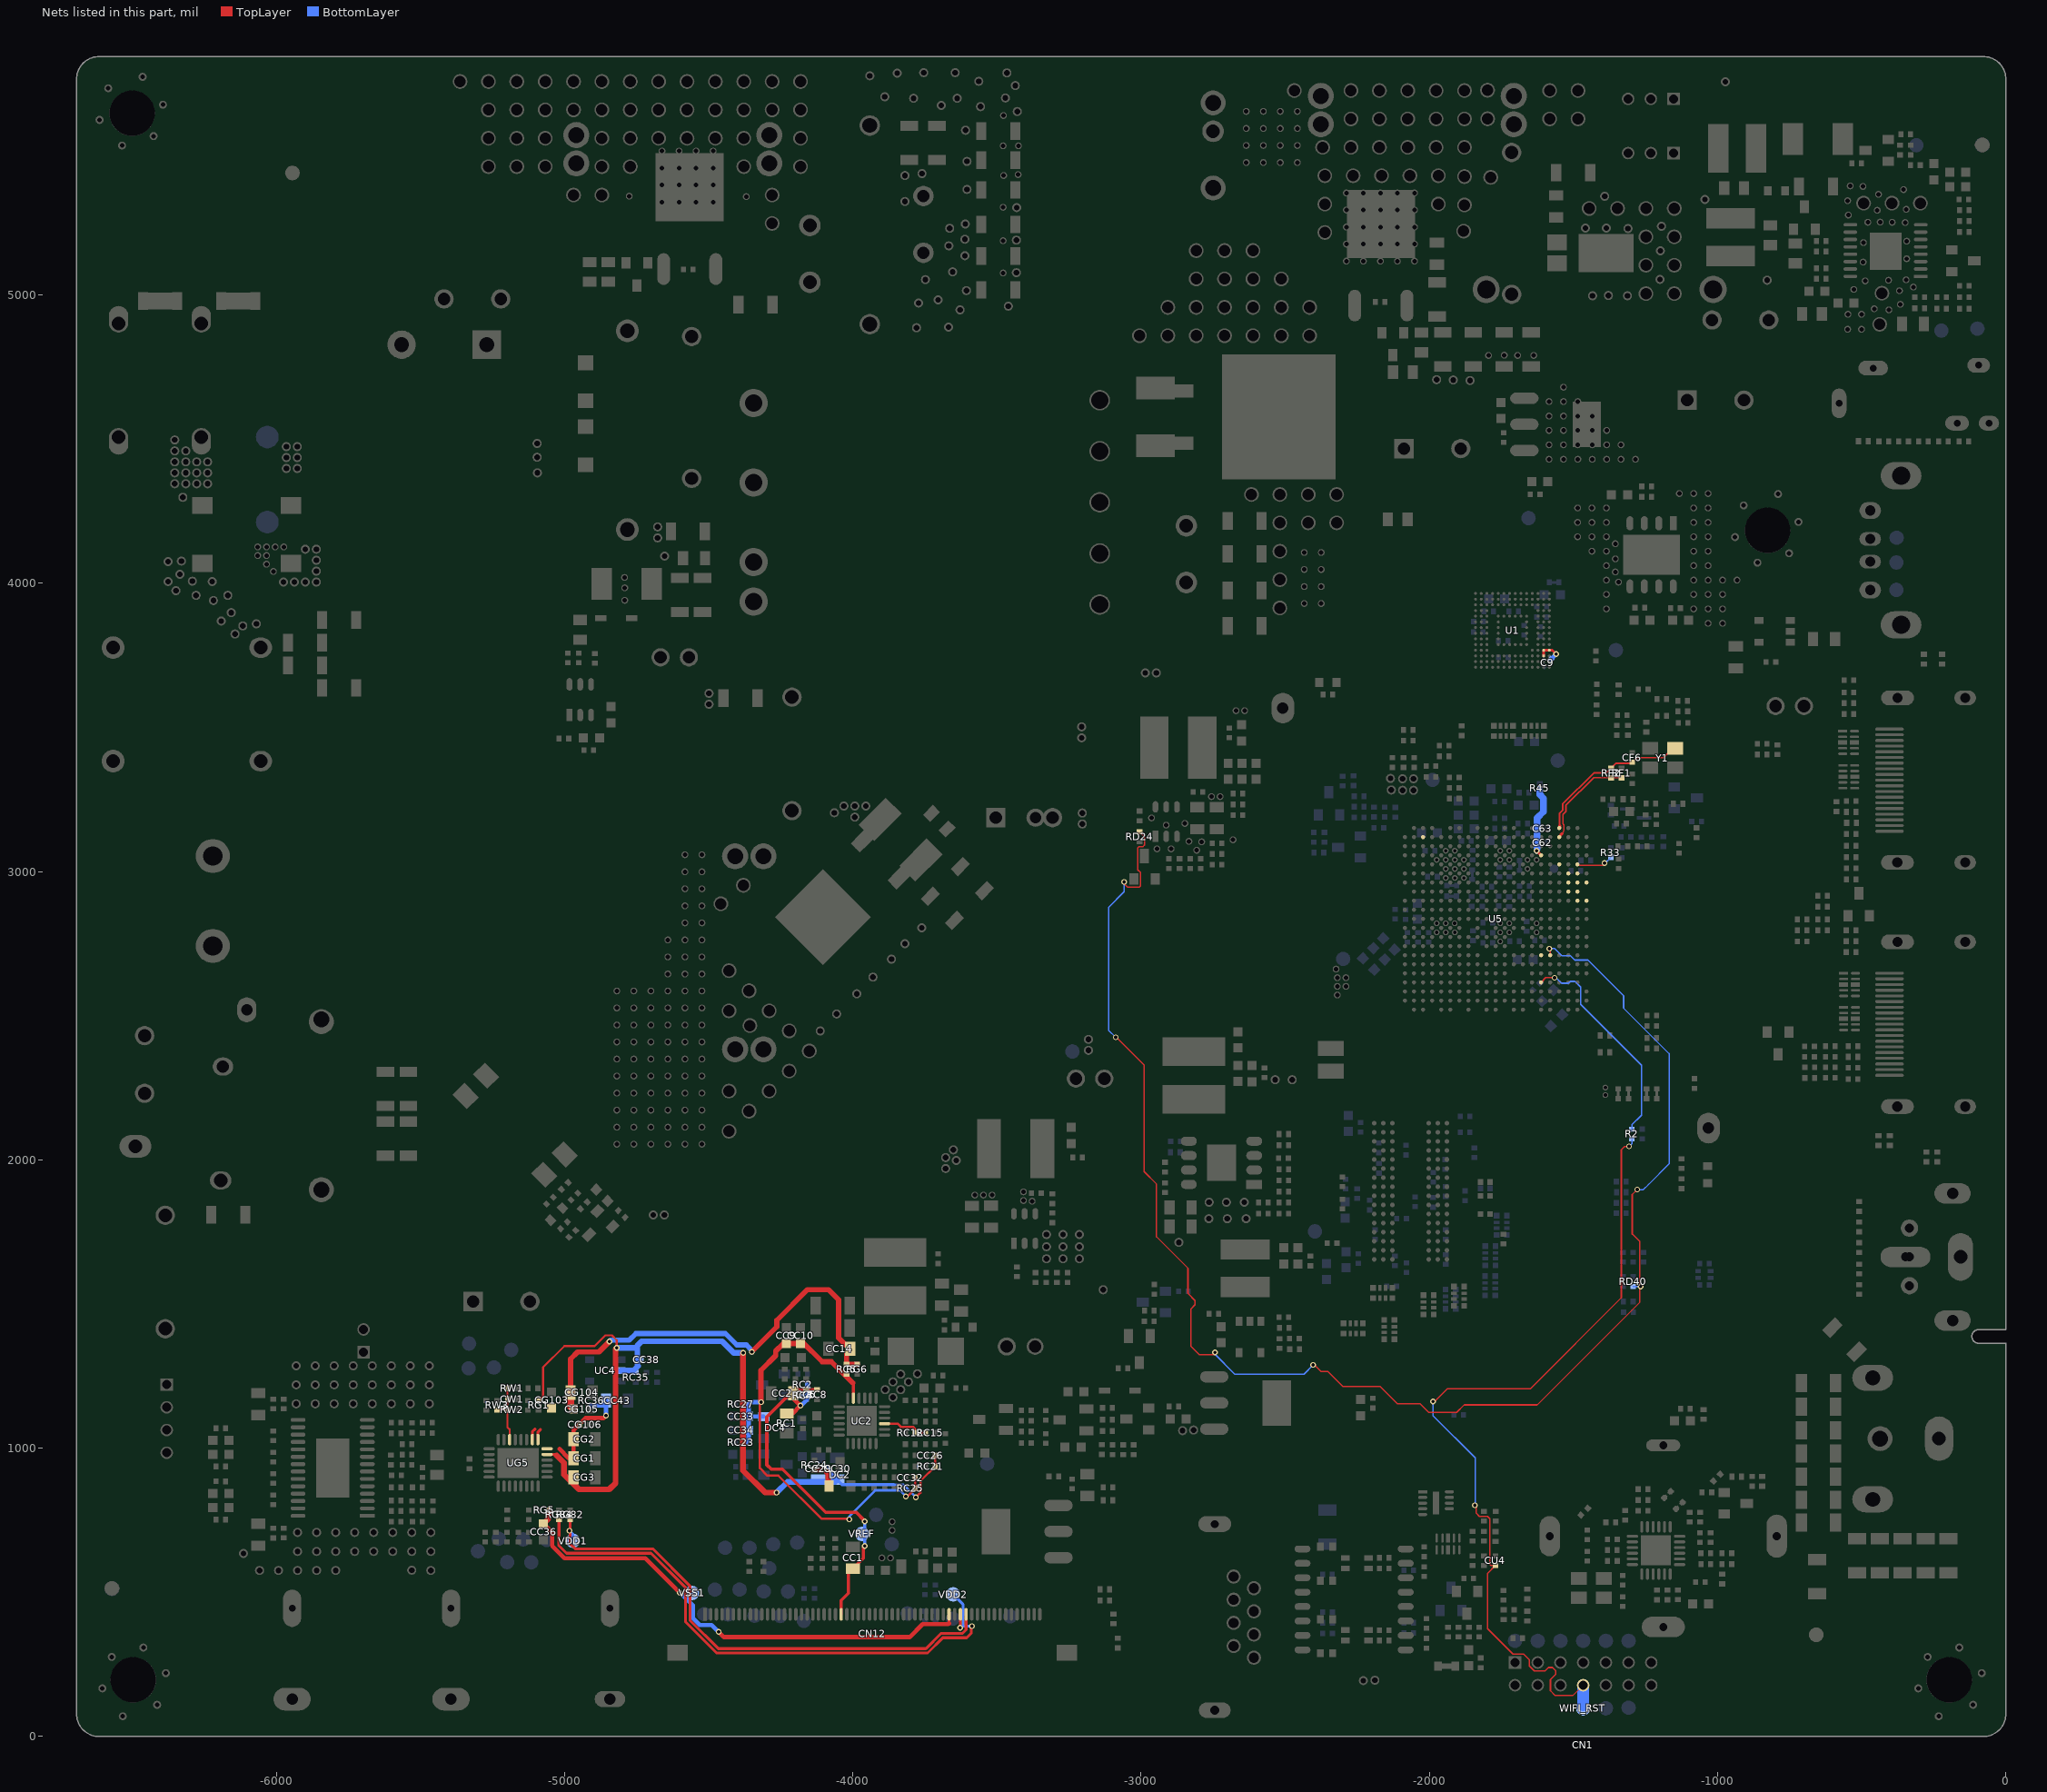
[diagram p0: the nets of this part, all layers, seen from the top]
# Altium PCB MISC84395.PcbDoc (part 24 of 26)
Units mil, origin at the board's own origin, x right, y up, seen from the top; angles counter-clockwise.
Board outline 6692.91 x 5826.77 mil, 2 copper layers (TopLayer, BottomLayer), stack 61.855 mil thick; 951 components, 565 nets, 4374 pads, 1804 vias.
Unrouted connection lines stored in the file: 1.

## Via types
v1: diameter 19.68, hole 11.81, TopLayer to BottomLayer, tented both sides, 1262 vias
v2: diameter 23.62, hole 15.75, TopLayer to BottomLayer, tented both sides, 524 vias
v3: diameter 31.5, hole 19.68, TopLayer to BottomLayer, tented both sides, 11 vias
v4: diameter 24, hole 16, TopLayer to BottomLayer, tented both sides, 6 vias
v5: diameter 19, hole 11.81, TopLayer to BottomLayer, tented both sides, 1 vias

## Nets (pads, with @x,y where several pads share a name; then routed paths per layer and width w, separated by ;. In a path a pad name is that pad's centre, name@x,y a point inside that pad or via, vN(x,y) a via of type N, cw(c..) or ccw(c..) an arc to the next point about the centre after c; other vN are vias at no path point) (continued)
VDD1: CN12.47 RG82.1 VDD1.1 | length 1792.2
  TopLayer w10: RG82.1@-4981,752.27 -4981,669 -4963,651 -4693.79,651 -4564.84,522.06 -4564.84,403.3 -4466.55,305 -3746.5,305 -3693.76,357.74 -3619.78,357.74 -3607.2,370.32 CN12.47@-3607.2,418.08
  BottomLayer w10: v1(-4983,714) -4971,702 VDD1.1@-4971,679
VDD2: CN12.46 RG84.1 VDD2.1 | length 2001
  TopLayer w10: RG84.1@-5019,752.27 -5019,661.75 -4993.25,636 -4700,636 -4579.84,515.84 -4579.84,397.08 -4472.76,290 -3740.29,290 -3687.54,342.74 -3604.76,342.74 -3589,358.5 -3589,381 v1(-3587,383) ; v1@-3626.89,377.59 CN12.46@-3626.89,418.08
  BottomLayer w10: VDD2.1@-3652,493 -3618,459 -3618,386.47 ; v1@-3626.89,377.59 -3621.47,383 v1(-3587,383)
  other v1: -3628,377.59
VDDI: C9.1 U1.C2 U1.D1 U1.D2 | length 98.1
  TopLayer w9.8: U1.C2@-1603.6,3747.97 U1.D2@-1603.6,3767.66 U1.D1@-1583.91,3767.66 -1573.52,3767.66 v1(-1560.21,3754.34)
  BottomLayer w9.8: v1@-1563.71,3750.84 v1(-1560.21,3754.34)
  BottomLayer w15: C9.1@-1577.17,3736.83 -1560.21,3753.8 v1(-1560.21,3754.34)
VDDP_EMMC: C62.2 C63.2 R45.2 R45.3 U5.V6 | length 245.6
  TopLayer w10: v1(-1628.24,3072.3) U5.V6@-1612.49,3056.56
  BottomLayer w19.68: v1(-1628.24,3072.3) -1626.27,3074.27 v1@-1626.27,3078.21
  BottomLayer w23.62: v1@-1626.27,3078.21 -1626.27,3185.65 -1603.63,3208.29 -1603.63,3253.71 -1617.27,3267.35 R45.2@-1617.27,3272.01 R45.2@-1617.27,3279.8
VDET1: CW1.2 RW1.2 RW2.2 RW3.2 UG5.6 | length 217.3
  TopLayer w7: RW3.2@-5236,1135.27 RW2.2@-5200,1135.27 ; RW1.2@-5197.73,1208 CW1.2@-5197.73,1170 RW2.2@-5197.73,1133 -5197.73,1072.11 -5190.53,1064.91 UG5.6@-5190.53,1029.71
VDIV: RC12.2 RC15.1 UC2.15 | length 162.9
  TopLayer w8: UC2.15@-3890,1085.08 -3845.08,1085.08 -3834,1074 -3791,1074 -3784.27,1067.27 RC12.2@-3784.27,1054 RC15.1@-3747.73,1054
VGA_B_IN_IC: U5.P3
VGA_COM_IN_IC: U5.R3
VGA_G_IN_IC: U5.P2
VGA_HS_IN_IC: U5.N1
VGA_R_IN_IC: U5.R2
VGA_VS_IN_IC: U5.N2
VGH: CC9.1 CC10.1 CC32.2 CC33.2 CC34.2 DC4.3 RC5.2 RC23.2 RC25.2 RC27.2 UC2.23 | length 1841.2
  TopLayer w8: v1@-4317.66,1164 -4318.5,1163.16 -4322,1159.66 -4322,931 -4296,905 -4258,905 -4108,755 -4014,755 v1(-4012,753) ; v1(-3816,833) -3810.06,833 -3784.26,858.8 CC32.2@-3784.26,898
  TopLayer w10: -4000.58,1226.57 -3998.27,1224.26 UC2.23@-3998.27,1173.66
  TopLayer w18: v1@-4318.5,1159.66 v1@-4318.5,1160.5 ; v1(-4317.66,1159.66) v1@-4318.5,1160.5 ; CC10.1@-4181,1363.19 CC9.1@-4231,1363.19 -4240.97,1363.19 -4267.37,1336.79 -4267.37,1321.51 -4318.5,1270.38 -4318.5,1163.16 v1@-4318.5,1160.5 ; CC10.1@-4181,1367.25 -4174.44,1367.25 CC10.1@-4175.37,1368.19 ; CC10.1@-4181,1368.19 CC10.1@-4175.37,1368.19 ; CC10.1@-4173.65,1368.19 CC10.1@-4174.65,1368.19 ; -4000.58,1226.57 -4074.01,1300 -4106.46,1300 CC10.1@-4174.65,1368.19 ; CC10.1@-4175.37,1368.19 CC10.1@-4174.65,1368.19
  BottomLayer w8: v1(-4012,753) -4012,764 -3922,854 -3836,854 -3816,834 v1(-3816,833)
  BottomLayer w15: RC23.2@-4372.27,1020.19 -4361.19,1031.27 ; CC34.2@-4361.19,1062.19 -4361.19,1031.27 ; v1@-4319.66,1160 -4352,1160 -4361.19,1150.81 -4361.19,1126 ; DC4.3@-4316.16,1110 DC4.3@-4318.77,1110 ; DC4.3@-4309.5,1110.19 CC33.2@-4361.19,1110.19 -4361.19,1126 ; -4361.19,1031.27 -4361.19,1126 ; DC4.3@-4318.77,1110 -4321.77,1110 -4320.27,1108.5 DC4.3@-4318.77,1110
VGHM: CC14.2 CG103.2 CG104.1 CG105.2 RC5.1 RG6.2 UG5.1 UG5.2@-5111.79,1029.71 | length 1665.2
  TopLayer w10: UG5.2@-5111.79,1029.71 -5111.79,1057.21 -5103,1066 ; UG5.1@-5092.1,1029.71 -5092.1,1056.9 -5084,1065
  TopLayer w18: -4979,1164 CG104.1@-4979,1193 -4979,1221 ; -4979,1245.18 -4979,1221 ; v1(-4844.5,1370) -4880.5,1334 -4954.5,1334 -4979,1309.5 -4979,1221 ; v1@-4350.54,1334.54 -4263.75,1421.33 -4263.75,1443.75 -4157.87,1549.63 -4083.63,1549.63 -4049,1515 -4049,1382.49 -4011.51,1345 CC14.2@-4009,1345 ; CC14.2@-4012.75,1341.25 -4011.51,1340 -4009,1340 -4022,1327 RC5.1@-4022,1290.73 RG6.2@-3985,1290.73
  TopLayer w25: CG105.2@-4979,1144 -4979,1164
  BottomLayer w18: v1(-4844.5,1370) -4839.5,1375 -4775.5,1375 -4752.5,1398 -4442,1398 -4402,1358 -4369.32,1358 -4350,1338.68 v1(-4350,1334)
VGL: CC26.2 CC29.1 CC30.1 CC38.1 CG3.1 DC2.1 RC21.2 RC24.2 RC35.2 RG1.1 UC4.2 UG5.27 | length 3244.4
  TopLayer w7: RG1.1@-5090,1165.73 -5074.08,1181.65 -5074.08,1280.91 -5000.49,1354.5 -4895.37,1354.5 -4859.18,1390.68 -4858.52,1391.34 -4835.66,1391.34 -4819,1374.68 v1(-4819,1348)
  TopLayer w8: v1(-3781,830) -3765,846 -3765,886.27 RC21.2@-3714.27,937 CC26.2@-3714.26,975
  TopLayer w10: UG5.27@-5060.61,978.53 -5023.67,978.53
  TopLayer w20: -5027.21,974.99 -5001.75,949.53 -5001.75,908.75 -4950,857 -4845,857 -4823,879 -4823,1344 v1(-4819,1348) ; v1(-4380.5,1331) -4380.5,922.78 -4303.85,846.13 v1(-4264.65,846.13) ; RC24.2@-4133,925 v1@-4101,925 ; v1(-4099,927) -4085.5,913.5 DC2.1@-4085.5,869
  BottomLayer w8: -3858,874 -3825,874 v1(-3781,830)
  BottomLayer w10: CC30.1@-4055,891 -4038,874 -3858,874
  BottomLayer w20: v1(-4819,1348) -4755.5,1348 ; UC4.2@-4804.87,1269.73 -4760.27,1269.73 -4744.81,1285.19 ; -4747.5,1287.88 -4747.5,1356 -4732.5,1371 -4453.18,1371 -4413.18,1331 v1(-4380.5,1331) ; v1@-4263.87,846.13 -4226.37,883.63 CC30.1@-4061.37,883.63 ; v1(-4099,927) -4091,927 -4055,891 CC30.1@-4061.37,891
VGPIN1: U5.Y19
VID0_OUT_IC: RD24.2 RD40.1 U5.G5 | length 5527.1
  TopLayer w5: v1@-3084.53,2424 -2989.5,2328.97 -2989.5,1959.16 -2946.5,1916.16 -2946.5,1733.36 -2837.5,1624.36 -2837.5,1537.03 -2812.66,1512.18 -2812.66,1497.82 -2827.5,1482.97 -2827.5,1353.73 -2798.27,1324.5 v1@-2744,1324.5 ; v1@-3059,2958 -3047,2946 -3005.9,2946 -3002.25,2949.65 -3002.25,2996.98 -3011.25,3005.98 -3011.25,3082.3 -3006.85,3086.69 -2993.27,3086.69 -2987.66,3092.3 -2987.66,3120.39 RD24.2@-3005,3137.73 ; v1(-2403,1289.16) -2398.68,1289.16 -2375.18,1265.66 -2351.59,1265.66 -2299.54,1213.61 -2169.89,1213.61 -2109.89,1153.61 -2031.42,1153.61 ; -2098.2,1153.61 -2031.42,1153.61 ; U5.G5@-1580.99,2710.1 v1@-1580.99,2732.09 ; -1296.17,1742.86 -1296.17,1879.83 v1@-1280,1896 ; -1295.67,1742.86 -1269.65,1716.84 -1269.65,1510.04 -1269.65,1506.62 -1625.92,1150.34 -1879.01,1150.34 -1905.01,1124.34 -2002.15,1124.34 -2031.42,1153.61
  BottomLayer w5: v1(-3088,2425) -3113,2450 -3113,2875.47 -3058.66,2929.82 v1@-3058.66,2963.66 ; v1(-2744,1332) -2744,1326.13 -2674.87,1257 -2435.16,1257 v1(-2403,1289.16) ; v1@-1581.65,2732.74 -1565.17,2732.74 -1540.94,2708.51 ; -1541.26,2708.51 -1540.94,2708.51 ; -1540.83,2708.4 -1540.94,2708.51 ; RD40.1@-1293.22,1561.31 v1@-1267.31,1561.31 ; v1@-1280,1896 v1@-1279,1896 ; v1(-1279,1897) -1257.8,1897 -1239.9,1914.9 -1168.3,1986.5 -1168.3,2368.3 -1326.3,2526.3 -1326.3,2569.45 -1449.86,2693.01 -1495.91,2693.01 -1511.41,2708.51 -1540.94,2708.51
  other v1: -1267,1561 -1583.65,2732.74 -3059,2964
VID1_OUT_IC: U5.G6
VREF: CC1.2 CC2.2 CC5.1 CN12.25 RC1.2 RC2.2 RC4.2 RC4.3 RC8.1 VREF.1 | length 1324.8
  TopLayer w11: CN12.25@-4040.27,423.98 -4040.27,471.73 -4015,497 -4015,579 -4008,586 CC1.2@-4002,586 ; CC1.2@-4000,571 CC1.2@-3996,571 ; CC1.2@-4000,581.97 -3963,618.97 v1@-3963,657 ; v1(-3959,746) v1@-3959,748.01
  TopLayer w12: CC2.2@-4221,1186 -4298.5,1108.5 -4298.5,942.6 -4283.03,927.13 -4243.83,927.13 -4094.29,777.59 -3987.87,777.59 -3959,748.72 v1@-3959,748.01
  TopLayer w15: RC1.2@-4229,1120.09 -4209.91,1120.09 v1(-4182,1148) -4207,1173 CC2.2@-4207,1191 ; CC2.2@-4196.27,1201.73 -4162,1201.73 RC8.1@-4124,1201.73
  BottomLayer w11: v1(-3959,661) v1(-3959,746)
  BottomLayer w15: v1@-4178.6,1148 -4157.24,1169.36 RC2.2@-4157.24,1221
VSS: CC43.2 CG1.1 CG2.1 CG106.2 RC36.2 UG5.28 | length 385
  TopLayer w15: -5017.89,997.49 -4985.39,965 CG1.1@-4969.03,965 CG2.1@-4969.03,1031 -4969.03,1062.62 -4927.31,1104.34 -4864.66,1104.34 v1(-4856.03,1112.97)
  BottomLayer w15: RC36.2@-4906.73,1147.99 -4902,1147.99 CC43.2@-4867.25,1147.99 ; v1(-4856.03,1112.97) CC43.2@-4856.03,1164.73
VSS1: CC36.1 CN12.44 RG5.1 VSS1.1 | length 1722.9
  TopLayer w10: -3666.26,392 CN12.44@-3666.26,418.08
  TopLayer w15: CC36.1@-5073,737.81 -5043,707.81 -5043,661 -5000.5,618.5 -4719.5,618.5 v1(-4600,499) ; v1(-4465.59,363.22) -4447.37,345 -3802.6,345 -3757.77,389.83 -3668.43,389.83 -3666.26,392
  TopLayer w18: CC36.1@-5073,737.81 -5055.27,755.54 RG5.1@-5055.27,785
  BottomLayer w15: v1(-4600,499) -4599,499 -4555,455 -4555,410.74 -4531.25,386.99 -4489.36,386.99 v1(-4465.59,363.22)
WIFI_HOST_WAKE_IC: U5.U4
WIFI_PWR_EN_IC: R33.2 U5.U2 | length 123.6
  TopLayer w5: U5.U2@-1486.5,3025.06 -1483.41,3021.97 v1@-1392.04,3021.97
  BottomLayer w5: v1@-1390.36,3029.3 R33.2@-1370.65,3049.01
  other v1: -1392.04,3029.3
WIFI_RESET: CN1.8 CU4.2 R2.1 WIFI_RST.1 | length 2891.7
  TopLayer w5: v1(-1987,1162) -1982,1162 -1937.36,1206.64 -1649.41,1206.64 -1334.17,1521.88 -1334.17,2035.14 -1322.64,2046.67 v1(-1306.95,2046.67) ; v1(-1842,802) -1838,798 -1838,775 -1826.63,763.63 -1798.05,763.63 -1790.34,755.92 -1790.34,597 -1786.61,593.26 CU4.2@-1771,593.26 -1798.25,566.01 -1798.25,374.11 -1710.03,285.89 -1672.89,285.89 -1653.17,266.17 -1653.17,244.66 -1636.09,227.59 -1598.95,227.59 -1587.18,239.36 -1572.82,239.36 -1562,228.54 -1562,215.49 -1580,197.49 -1580,159 -1563,142 -1502.54,142 CN1.8@-1466.54,178
  BottomLayer w5: v1(-1987,1162) -1987,1112.43 -1841,966.43 v1@-1841,802 ; v1(-1306.95,2046.67) -1297.65,2055.98 R2.1@-1297.65,2071.13
  BottomLayer w40: WIFI_RST.1@-1466.48,108 CN1.8@-1466.48,177.94
WIFI_RESET_IC: R2.2 U5.D6 | length 752.5
  TopLayer w4: U5.D6@-1612.49,2615.61 -1595.96,2632.14 v1@-1566.95,2632.14
  BottomLayer w5: v1@-1560.65,2631.84 -1541.47,2612.66 -1517.72,2612.66 -1511.28,2619.1 -1495.07,2619.1 -1474.91,2598.94 -1474.91,2539.14 -1264.3,2328.54 -1264.3,2154.9 -1297.65,2121.56 R2.2@-1297.65,2104.6
  other v1: -1565.49,2631.6
XTALI_IN_IC: CF6.1 RF2.1 U5.AA4 Y1.3 | length 558.1
  TopLayer w6: -1548.65,3159.14 -1548.65,3201.3 -1537.65,3212.3 -1537.65,3232.7 -1537.56,3232.79 -1537.56,3233.71 -1429.53,3341.74 -1386.38,3341.74 -1352.38,3375.74 -1299.91,3375.74 -1280.45,3395.2 -1188.68,3395.2 -1156.22,3427.67 Y1.3@-1148.03,3427.67
  TopLayer w10: U5.AA4@-1549.5,3151.04 U5.AA4@-1547.65,3152.89 ; -1547.65,3159.14 U5.AA4@-1547.65,3152.89 ; U5.AA4@-1547.47,3153.07 U5.AA4@-1547.65,3152.89
XTALO_OUT_IC: RF1.2 RF2.2 U5.Y4 | length 355.6
  TopLayer w5: U5.Y4@-1549.5,3119.55 U5.Y4@-1549.5,3121.71 ; -1539.59,3131.61 ccw(c-1553.7,3145.72) -1533.75,3145.72 -1533.75,3160.16 ccw(c-1540.23,3160.16) -1535.65,3164.74 cw(c-1533.23,3167.15) -1536.65,3167.15 -1536.65,3181.85
  TopLayer w6: -1536.65,3181.85 -1536.65,3197.74 -1526.65,3207.74 -1526.65,3228.15 -1526.56,3228.23 -1526.56,3229.15 -1429.97,3325.74 -1334.38,3325.74 RF1.2@-1333.65,3325.01
  TopLayer w10: U5.Y4@-1549.5,3119.55 -1549.5,3121.71 -1539.59,3131.61
YPP_B_IN_IC: U5.R1
YPP_R_IN_IC: U5.T2
YPP_Y_IN_IC: U5.T3
pads on no net: "Conformal Coating.0" AI_V.0 AI_V.1 AI_V.2 AVE1.0 AVH1.0 AVH2.0 AVH2.14 AVI1.0 AVO1.0 AVO2.0 AVU2.0 AVU2.1@-470.76,4074.8 AVU2.2@-470.76,4153.54 BB101.35 BB101.36 BB801.35 BB801.36 CB114.1@-3755,5146.15 CB114.1@-3755,5343 CB116.0 CB118.0 CB120.41 CB120.42 CB815.43 CB815.44 CN1.0 CN2.0 CN12.1 CN12.20 CN12.24 CN12.26 CN12.29 CN12.31 CN12.32 CN12.36 CN12.37 CN12.40 CN12.43 CN12.45 CN12.48 CN12.50 CN12.53 CN12.60 CNA1.0 CNB1.109 CNB1.110 CNB2.0 CNB822.0 CNB832.0 CT01.2@-1133,801 CT05.2@-1174,839 CXB1.77 CXB1.78 CYB1.61 CYB2.61 CYB3.61 CYB4.61 DB106.0 DB106.1 DB801.0 DB801.1 DE2.2 DE2.4 DE2.5 DE2.6 DE2.8 DE2.10 DE2.EPAD@-1977,787 DE2.EPAD@-1977,832.27 DE2.EPAD@-1977,832.28 EA1.0 EB1.1@-5269.73,4827.43 EB1.1@-5565.01,4827.43 EB101.0 EB101.1@-3307.15,3187 EB101.1@-3504,3187 EB102.1@-3366.2,3187 EB102.1@-3504,3187 EB104.0 EB104.1@-1891.05,4467 EB104.1@-2087.9,4467 EB106.0 EB801.0 EB801.1@-908.79,4635 EB801.1@-1105.65,4635 EC1.0 EC1.5 EC1.6 ED1.0 ED1.5 ED1.6 EU2.0 FB1.4 FB1.5 GD1.0 GD2.0 GD3.0 GD4.0 H1.0 H2.0 H3.0 H4.0 HS3.2@-1031.98,2110.2 HS3.2@-2508.35,3566.89 LB801.1@-2750.11,5370.72 LB801.1@-2750.11,5666 LB802.3 LB802.4 LCB1.4@-6054,3383 LCB1.4@-6054,3776.7 LCB1.4@-6565.81,3383 LCB1.4@-6565.81,3776.7 M1.0 M2.0 M3.0 M4.0 M5.0 M6.0 MAC.0 Manufacture_Info.0 MOVB1.2@-6193,1929 MOVB1.2@-6488.28,2047.11 NTCB1.2@-6184.97,2323.57 NTCB1.3 PT1.0 RB148.69 RFT1.0 S/N1.0 S/N2.0 TB101.2 TB101.3@-4344.32,4349.41 TB101.6@-4344.32,4073.82 TB101.7@-4344.32,3936.02 TB101.12 U1.A1 U1.A7 U1.A9 U1.A10 U1.A11 U1.A12 U1.A13 U1.A14 U1.B1 U1.B8 U1.B9 U1.B10 U1.B11 U1.B12 U1.B13 U1.B14 U1.C7 U1.C8 U1.C9 U1.C10 U1.C11 U1.C12 U1.C13 U1.C14 U1.D12 U1.D13 U1.D14 U1.E5 U1.E8 U1.E9 U1.E10 U1.E12 U1.E13 U1.E14 U1.F10 U1.F12 U1.F13 U1.F14 U1.G3 U1.G10 U1.G12 U1.G13 U1.G14 U1.H1 U1.H2 U1.H3 U1.H12 U1.H13 U1.H14 U1.J1 U1.J2 U1.J3 U1.J12 U1.J13 U1.J14 U1.K1 U1.K2 U1.K3 U1.K6 U1.K7 U1.K10 U1.K12 U1.K13 U1.K14 U1.L1 U1.L2 U1.L3 U1.L12 U1.L13 U1.L14 U1.M3 U1.M7 U1.M10 U1.M11 U1.M12 U1.M13 U1.M14 U1.N1 U1.N3 U1.N6 U1.N8 U1.N11 U1.N12 U1.N13 U1.N14 U1.P1 U1.P2 U1.P7 U1.P10 U1.P12 U1.P13 U1.P14 U5.B6 U5.C7 U5.F4 U5.H20 U5.H21 U5.J19 U5.J20 U5.K21 U5.N11 U5.N12 U5.N13 U5.N14 U5.N15 U5.N16 U5.P11 U5.P12 U5.P13 U5.R11 U5.R13 U5.Y16 UA1.0 UA1.13 UB801.0 UE1.4 UE1.5 UE1.12 UE1.13 UG5.2@-5111.79,974.98 UG5.2@-5161,974.97 UG5.2@-5210.21,974.98 UG5.3@-5111.79,923.02 UG5.3@-5161,923 UG5.3@-5210.21,923.02 UG5.20 UG5.21 UG5.22 UG5.24 UM1.J1 UM1.J9 UM1.L1 UM1.L9 UT2.5 UT2.7 UT2.8 UT2.18 XXXXXX.0 XXXXXXXXXXXXXXXX.0 用于U5上.0
copper on no net: | length 3402.8
  TopLayer w5: -2055.03,2771.5 -2053.43,2773.09 ; 3734.7,438.69 3734.7,517.43 ; 3183.8,438.69 3183.8,517.43 3915.83,517.43 3915.83,438.69 3183.8,438.69
  BottomLayer w5: 3734.7,220.84 3734.7,299.58 ; 3183.8,220.84 3915.83,220.84 3915.83,299.58 3183.8,299.58 3183.8,220.84

## Polygon pours and split planes (outlines as drawn)
GND on BottomLayer "5mil" (solid, remove dead copper, pour order 1046): -723,5173 -723,5788 -684,5827 -134,5827 -42,5735 -42,5005 -110,4937 -227,4937 -322,4842 -648,4842 -717,4911 -717,5038
GND on BottomLayer "5" (solid, remove dead copper, pour order 1031): -4757,774 -4754,771 -4754,295 -4754,292 -4629,167 -4593,203 -3955,203 -3955,470 -3808,617 -3740,685 -3740,942 -4603,942 -4769,776
D_QB801 on BottomLayer "5mil" (solid, remove dead copper, pour order 1045): -2950,5736 -2984,5702 -2984,5493 -2946,5455 -2679,5455 -2216,4992 -1917,4992 -1906,5003 -1906,5104.7 -1871.67,5140 -1576,5140 -1541,5175 -1541,5398 -1494,5445 -1423,5445 -1393,5475 -1393,5706 -1423,5736 -2673,5736
GND on BottomLayer "5mil" (solid, remove dead copper, pour order 1060): -6195,5826.77 -6631.23,5826.77 -6690,5768 -6690,5042 -6660,5012 -6225,5012 -6075,5162 -6007,5230 -6007,5481 -6007,5762.77 -6071,5826.77
D_QB101 on BottomLayer "5mil" (solid, remove dead copper, pour order 1044): -4711,5829 -5355,5829 -5387,5797 -5387,5489 -5232,5334 -5142,5244 -5093,5195 -5022,5195 -4954,5195 -4913,5195 -4648,4930 -4648,4861 -4648,4782 -4625,4759 -4501,4759 -4348,4912 -4348,5104 -4276,5176 -4262,5190 -4184,5190 -4100,5190 -4079,5211 -4067,5223 -4067,5242 -4067,5756 -4138,5827
NetDB106_K on BottomLayer "5mil" (solid, remove dead copper, pour order 1043): -3655,5559 -3860,5559 -3883,5536 -3946,5536 -3975,5565 -3975,5785 -3934,5826 -3598,5826 -3536,5764 -3536,5353 -3560,5329 -3615,5329 -3627,5341 -3627,5531
GND on BottomLayer "5" (solid, remove dead copper, pour order 1036): -1319,1374 -821,1374 -434,1761 -358,1837 -358,2016 -358,3334 -769,3745 -1397,4373 -1735,4373 -1800,4373 -1852,4321 -2127,4046 -2127,3767 -2135,3767 -2296,3606 -2432,3470 -2502,3470 -2533,3470 -2558,3495 -2565,3502 -2565,3528 -2565,3559 -2596,3590 -2622,3616 -2692,3616 -2948,3616 -3093,3471 -3212,3352 -3251,3352 -3358,3245 -3358,3048 -3358,2240.27 -3610.97,1987.3 -3654.3,1943.97 -3689.97,1943.97 -3738,1992 -4013.41,2267.41 -4018.5,2267.41 -4032.59,2267.41 -4196,2104 -4647,1653 -4647,1623 -4009,1623 -3597,1211 -3152,766 -2271,766 -1958,766 -1912,720 -1816,624 -1325,624 -1312,624 -1202,734 -1198,738 -1198,1348
GND on BottomLayer "12" (solid, remove dead copper, pour order 1041): -6692.91,1435 -6692.91,46.91 -6673,27 -6646,0 -6559,0 -46,0 -23,23 0,46 0,78.74 0,4760 -17,4777 -34,4794 -95,4794 -500,4794 -525,4769 -564,4730 -564,4618 -564,4586 -652,4498 -705,4445 -856,4445 -1089,4445 -1144,4500 -1372,4728 -1560,4728 -1738,4728 -1781,4685 -1794,4672 -1794,4599 -1794,4420 -1889,4325 -2175,4039 -2175,3972 -2175,3820 -2200,3795 -2240,3755 -2456,3755 -2975,3755 -3034,3696 -3223,3507 -3223,3435 -3223,3395 -3238,3380 -3245,3380 -3252,3380 -3256,3384 -3451,3189 -3451,3131 -3451,2969 -3699,2721 -4566,1854 -4612,1854 -4775,1854 -4865,1854 -4903,1816 -4974,1745 -5119,1745 -5316,1745 -5497,1564 -5617,1444 -6147,1444 -6677.91,1444 -6692.91,1429
RFGND on BottomLayer "12" (solid, remove dead copper, pour order 1033): -628,1276 -515,1389 -1,1389 -1,654 -12,643 -597,643 -628,674
D_QB801 on TopLayer "5mil" (solid, remove dead copper, pour order 1051): -2104,5825 -1441,5825 -1376,5760 -1376,5529 -1413,5492 -1609,5492 -1627,5474 -1627,5157 -1643,5141 -1760,5141 -1878,5141 -1952,5067 -1961,5058 -2101,5058 -2310,5058 -2704,5452 -2779,5452 -3013,5452 -3036,5475 -3036,5760.77 -2970,5826.77 -2165,5826.77
VBL on TopLayer "5mil" (solid, remove dead copper, pour order 1059): -2759,4686 -2825,4752 -2866,4752 -3015,4752 -3041,4778 -3041,5262 -3012,5291 -2627,5291 -2352,5016 -2352,4925 -2224,4797 -2224,3836 -2250,3810 -2588,3810 -2620,3842 -2620,4231.99 -2759,4370.99 -2759,4437
GND on TopLayer "5mil" (solid, remove dead copper, pour order 1058): -3390.42,3036.58 -3426,3072.16 -3426,3211 -3426,3269 -3412,3283 -3262,3283 -3253,3274 -3238.19,3259.19 -3238.19,3152.77 -3238.19,3096.81 -3259,3076
D_QB101 on TopLayer "5mil" (solid, remove dead copper, pour order 1057): -5395,5361 -5395,5790 -5357,5828 -4141,5828 -4068,5755 -4068,5330 -4039,5301 -3971,5301 -3902,5232 -3902,4877 -3920,4859 -4001,4859 -4021,4879 -4021,5147 -4069,5195 -4291,5195 -4323,5227 -4349,5253 -4450,5253 -4998,5253 -5059,5314 -5080,5335 -5120,5335 -5369,5335
VBRIDGE on TopLayer "5mil" (solid, remove dead copper, pour order 1056): -3789,5216 -3732,5216 -3673,5275 -3666,5282 -3570,5282 -3544,5282 -3537,5275 -3537,4975 -3582,4930 -3612,4900 -3655,4857 -3758,4857 -3795,4857 -3806,4868 -3806,5199
NetCB114_1 on TopLayer "5mil" (solid, remove dead copper, pour order 1055): -3709,5504 -3831,5504 -3841,5494 -3841,5316 -3819,5294 -3724,5294 -3672,5346 -3672,5496 -3680,5504
NetDB106_K on TopLayer "5mil" (solid, remove dead copper, pour order 1054): -3639,5559 -3860,5559 -3883,5536 -3946,5536 -3975,5565 -3975,5785 -3934,5826 -3598,5826 -3535,5763 -3535,5329 -3553,5329 -3558,5334 -3558,5529 -3588,5559
SGND on TopLayer "5mil" (solid, remove dead copper, pour order 1053): -5759,4652 -5485,4652 -5438,4699 -5438,4881 -5346,4973 -5346,5054 -5362,5054 -5430,5122 -5441,5122 -5463,5100 -5634,4929 -5634,4802.77
NetCB118_2 on TopLayer "5mil" (solid, remove dead copper, pour order 1052): -2727,4262 -2696,4262 -2677,4243 -2661,4227 -2661,4183 -2661,3836 -2674,3823 -3015,3823 -3039,3847 -3039,4164 -3015,4188 -2978,4188 -2940,4150 -2910,4120 -2853,4120 -2795,4120 -2772,4143 -2772,4245 -2755,4262
L on TopLayer "5mil" (solid, remove dead copper, pour order 1050): -6377,4525 -6377,4318 -6299,4240 -6221,4240 -6219,4242 -6219,4529 -6226,4536 -6365,4536 -6374,4527
N on TopLayer "5mil" (solid, remove dead copper, pour order 1049): -6535,4537 -6642,4537 -6690,4489 -6690,3973 -6665,3948 -6307,3948 -6222,3863 -6098,3739 -6016,3739 -6004,3751 -6004,3825 -6038,3859 -6221,4042 -6221,4081 -6221,4092 -6227,4098 -6342,4098 -6512,4268 -6512,4446 -6512,4520 -6529,4537
GND on TopLayer "5mil" (solid, remove dead copper, pour order 1048): -6691,5176 -6691,5782 -6645,5828 -6042,5828 -6003,5789 -6003,4955 -6051,4907 -6090,4907 -6111,4928 -6111,5001 -6136,5026 -6260,5026 -6296,4990 -6310,4976 -6310,4911 -6323,4898 -6375,4898 -6386,4909 -6386,4996 -6420,5030 -6656,5030 -6692.56,5066.56
SGND on TopLayer "5mil" (solid, remove dead copper, pour order 1047): -4991,3806 -5077,3806 -5090,3793 -5090,3518 -5077,3505 -5022,3505 -5008,3519 -5004.1,3522.9 -4982.89,3522.9 -4982.89,3524.11 -4976,3531 -4976,3564 -4965,3575 -4903,3575 -4890,3562 -4890,3475.62 -4878.68,3464.3 -4878.68,3441.65 -4849.35,3441.65 -4823,3468 -4823,3527 -4828,3532 -4849,3532 -4862,3545 -4862,3572 -4883,3593 -4886,3596 -4921,3596 -4978,3596 -5004,3622 -5015.49,3633.49 -5015.49,3647 -5015.49,3737.17 -4991.77,3760.89
GND on TopLayer "5" (solid, remove dead copper, pour order 1037): -2097.5,3126.49 -2129.83,3158.82 -2168,3158.82 -2399.58,3158.82 -2532.92,3025.48 -2699.4,2859 -3451.66,2859 -3472.48,2838.17 -4789,1521.66 -4789,1406 -4789,811 -4695,717 -4504,526 -4504,490 -4504,453 -4460,409 -4459,410 -4054,410 -4054,438 -4075,459 -4081.7,465.7 -4143.7,465.7 -4146.7,465.7 -4156,475 -4159,478 -4159,530 -4159,721 -4189,751 -4242.63,804.63 -4319.63,804.63 -4411,896 -4411,925 -4411,1365.09 -4265.95,1510.13 -3295.09,2481 -2900,2481 -2585.25,2481 -2440.12,2626.13 -2329.24,2737.01 -2110.14,2737.01 -2090.97,2756.18 -2080.17,2766.98 -2080.17,2823.39
GND on TopLayer "5mil" (solid, remove dead copper, pour order 1038): -2072.14,2725.84 -1757.41,2725.84 -1731.68,2700.11 -1641.39,2609.83 -1641.39,2575.33 -1640.28,2575.33 -1620.23,2555.28 -1390.66,2325.71 -1390.66,2246.96 -1390.66,2142.9 -1389.5,2141.74 -1389.5,1573.1 -1542.73,1419.87 -1664.93,1297.67 -1706.79,1297.67 -2300.8,1297.67 -2353.97,1350.84 -2353.97,1406.29 -2353.97,2275.26 -2198.97,2430.26 -2195.58,2433.65 -2195.58,2457.41 -2195.58,2618.08 -2142.4,2671.26 -2103.56,2710.1 -2088.87,2710.1
GND on TopLayer "5" (solid, remove dead copper, pour order 1032): -2047,287 -2041,281 -1995,281 -1952,324 -1952,365 -1952,542 -1894,600 -1877,617 -1877,655 -1877,803 -1852,828 -1847,833 -1832,833 -1531,833 -1487,877 -1487,901.3 -1533.39,947.69 -1540.08,941 -1644,941 -1988,941 -2063,866 -2091,838 -2091,732 -2091,692 -2047,648
GND on TopLayer "5" (solid, remove dead copper, pour order 1035): -2116,3182.1 -1423,3182.1 -1423,3044 -1423,2490.11 -1582.89,2490.11 -2117,2490.11 -2117,2582 -2117,3182.1 -2115,3182.1
GND on TopLayer "5" (solid, remove dead copper, pour order 1040): -389,1938 -214,2113 -214,4048 -290,4124 -290,2130 -381,2039 -463,2039 -514,1988 -514,1938
GND on TopLayer "5" (solid, remove dead copper, pour order 1039): -643,3527 -819,3351 -819,3130 -900,3049 -1230,3049 -1381.92,2897.08 -1433.86,2897.08 -1433.86,2645.86 -1475.14,2645.86 -1639,2482 -1639,2460 -1445,2266 -1381,2266 -1367,2252 -1367,2130 -1213,1976 -1213,1862 -1206,1862 -1127,1783 -1127,1718 -1229,1616 -1229,1569 -1215,1555 -1193,1555 -1070,1678 -1070,1803.25 -1063,1810.25 -1061.75,1809 -1002,1809 -990,1821 -990,1887 -1017,1914 -1017,2040 -1188,2211 -1188,2274 -1227.49,2313.49 -1227.49,2344 -1214.63,2356.87 -985.87,2356.87 -795,2166 -795,1739 -890,1644 -890,1601.9 -1533.39,958.51 -1533.39,812.39 -1513,792 -1080,1225 -1009,1225 -674,1560 -674,2197 -922,2445 -1057,2445 -1101,2489 -1101,2507 -1091,2517 -718,2517 -624,2423 -468,2423 -461,2430 -461,2670 -469,2678 -574,2678 -629,2733 -1194,2733 -1213,2752 -1213,2760 -1140,2833 -811,2833 -603,3041 -603,3251 -594,3260 -475,3260 -462,3273 -462,3511.5 -446.5,3527
GND on TopLayer "12" (solid, remove dead copper, pour order 1042): -9,4706 -9,41 -50,0 -6640,0 -6692.91,52.91 -6692.91,1275.09 -6609,1359 -5333,1359 -5185,1507 -4920,1507 -3174,3253 -3174,3593 -3012,3755 -2634,3755 -2597,3718 -2451,3718 -2395,3662 -2186,3662 -2172,3676 -2172,4048 -1955,4265 -1775,4265 -1759,4281 -1759,4448 -1662,4545 -1662,4627 -1603,4686 -591,4686 -571,4706
RFGND on TopLayer "12" (solid, remove dead copper, pour order 1034): -628,1275 -528,1375 -1,1375 -1,654 -12,643 -580,643 -628,691